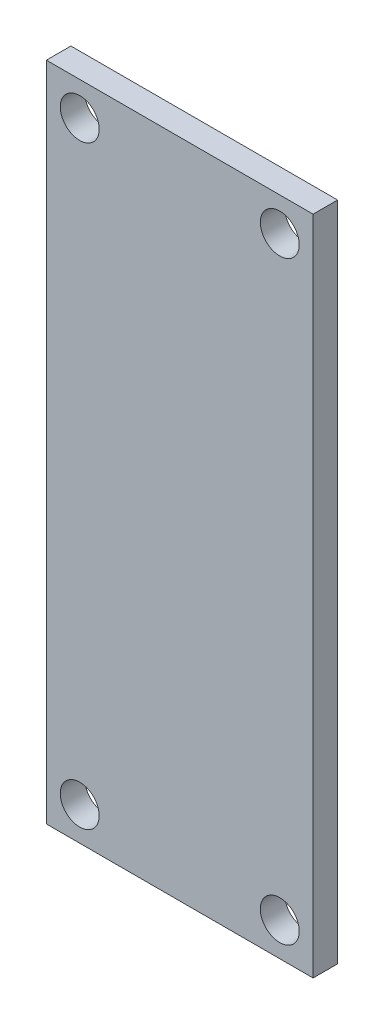
from build123d import *

# Parameters (mm, degrees)
SKETCH1_W           = 152.4
SKETCH1_H           = 377.95
SKETCH1_R           = 11.125
BOSS_EXTRUDE1_DEPTH = 14


with BuildPart() as part:
    # Sketch1 → Boss-Extrude1 (new body)
    with BuildSketch(Plane.XY):
        Rectangle(SKETCH1_W, SKETCH1_H)
        with Locations((-57.15, 169.8625)):
            Circle(SKETCH1_R, mode=Mode.SUBTRACT)
        with Locations((57.15, 169.8625)):
            Circle(SKETCH1_R, mode=Mode.SUBTRACT)
        with Locations((57.15, -169.8625)):
            Circle(SKETCH1_R, mode=Mode.SUBTRACT)
        with Locations((-57.15, -169.8625)):
            Circle(SKETCH1_R, mode=Mode.SUBTRACT)
    extrude(amount=BOSS_EXTRUDE1_DEPTH)


solid = part.part
